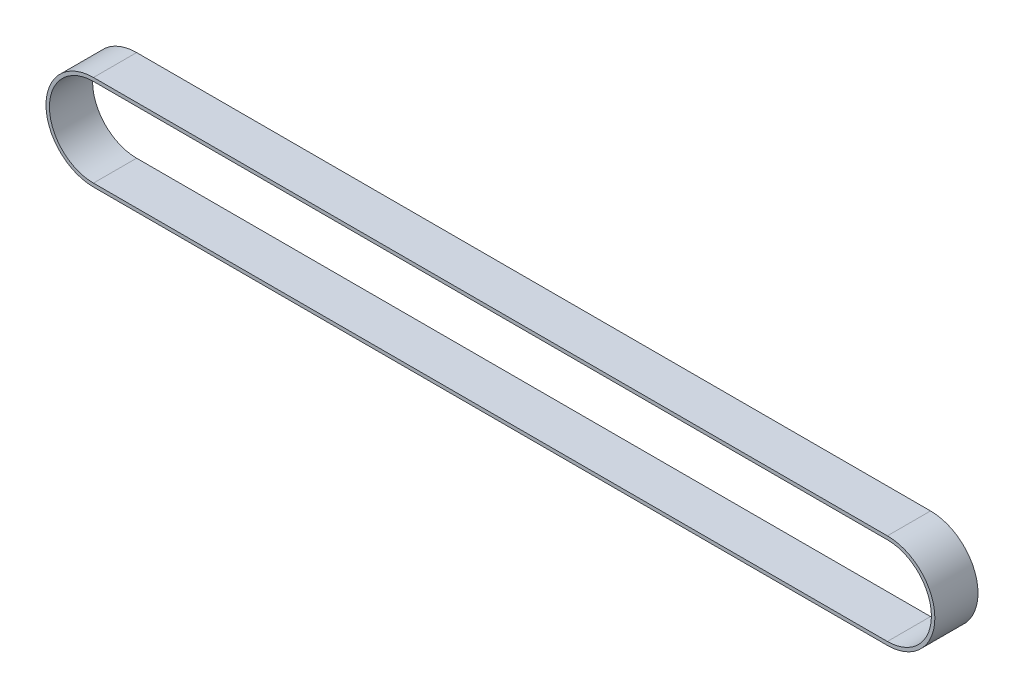
from build123d import *

# Parameters (mm, degrees)
EXTRUDE_1_DEPTH = 25


with BuildPart() as part:
    # 草图1 → 拉伸-薄壁1 (new body)
    with BuildSketch(Plane.XY):
        with BuildLine():
            Line((230, -27.5), (-230, -27.5))
            ThreePointArc((-230, -27.5), (-257.5, 0), (-230, 27.5))
            Line((-230, 27.5), (230, 27.5))
            ThreePointArc((230, 27.5), (257.5, 0), (230, -27.5))
        make_face()
        with BuildLine():
            Line((230, -25.5), (-230, -25.5))
            ThreePointArc((-230, -25.5), (-255.5, 0), (-230, 25.5))
            Line((-230, 25.5), (230, 25.5))
            ThreePointArc((230, 25.5), (255.5, 0), (230, -25.5))
        make_face(mode=Mode.SUBTRACT)
    extrude(amount=EXTRUDE_1_DEPTH)


solid = part.part
